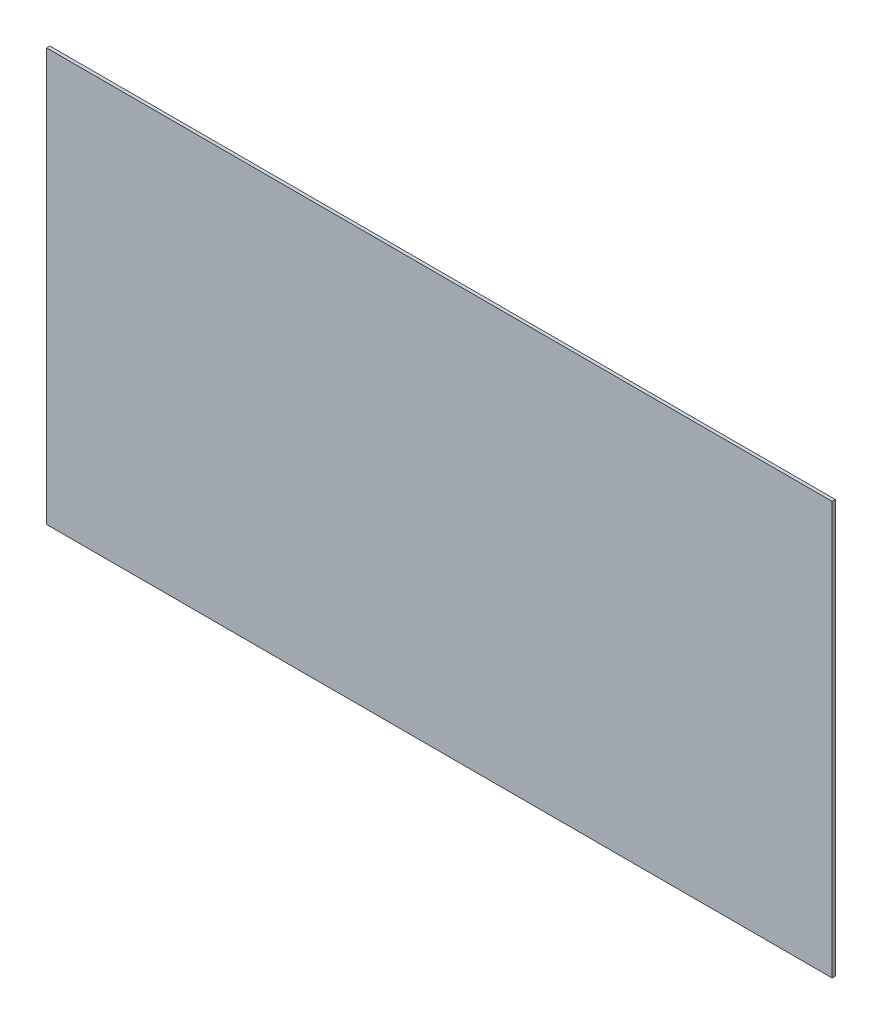
SolidWorks part; units mm, degrees
material "PMMA(有机玻璃)"
ref_plane "前视" through (0, 0, 0) normal (0, 0, 1) x (1, 0, 0)
ref_plane "上视" through (0, 0, 0) normal (0, 1, 0) x (1, 0, 0)
ref_plane "右视" through (0, 0, 0) normal (1, 0, 0) x (0, 0, -1)
sketch "草图1" plane through (0, 0, 0) normal (0, 0, 1) x (1, 0, 0)
  line L1 (-608, 319.5) -> (608, 319.5)
  line L2 (-608, 319.5) -> (-608, -319.5)
  line L3 (-608, -319.5) -> (608, -319.5)
  line L4 (608, 319.5) -> (608, -319.5)
  line L5 (-608, 319.5) -> (608, -319.5) construction
  line L6 (-608, -319.5) -> (608, 319.5) construction
  point P0 (0, 0)
  dimension "D1" = 639
  dimension "D2" = 1216
extrude "凸台-拉伸1" add sketch "草图1" along normal blind 5
